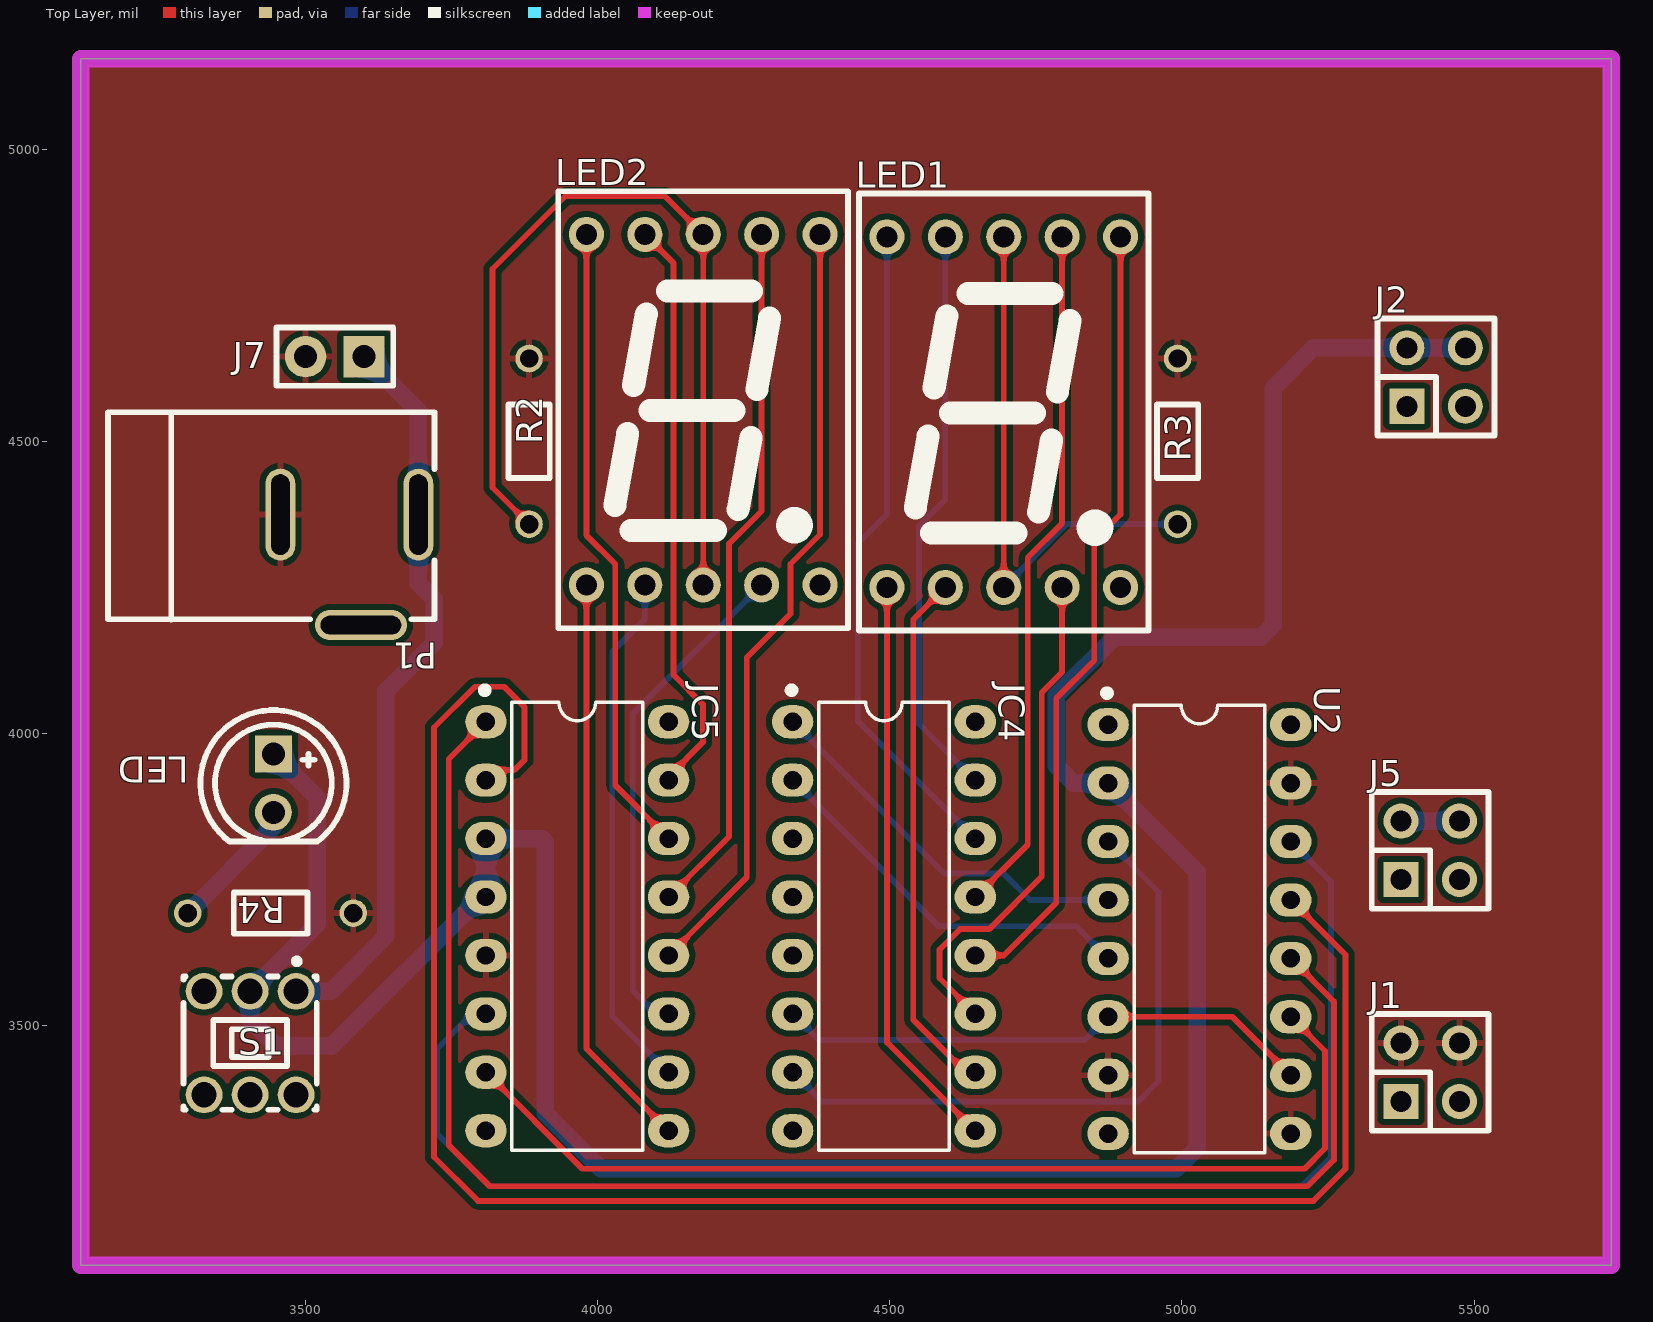
[diagram p0: Top Layer view]
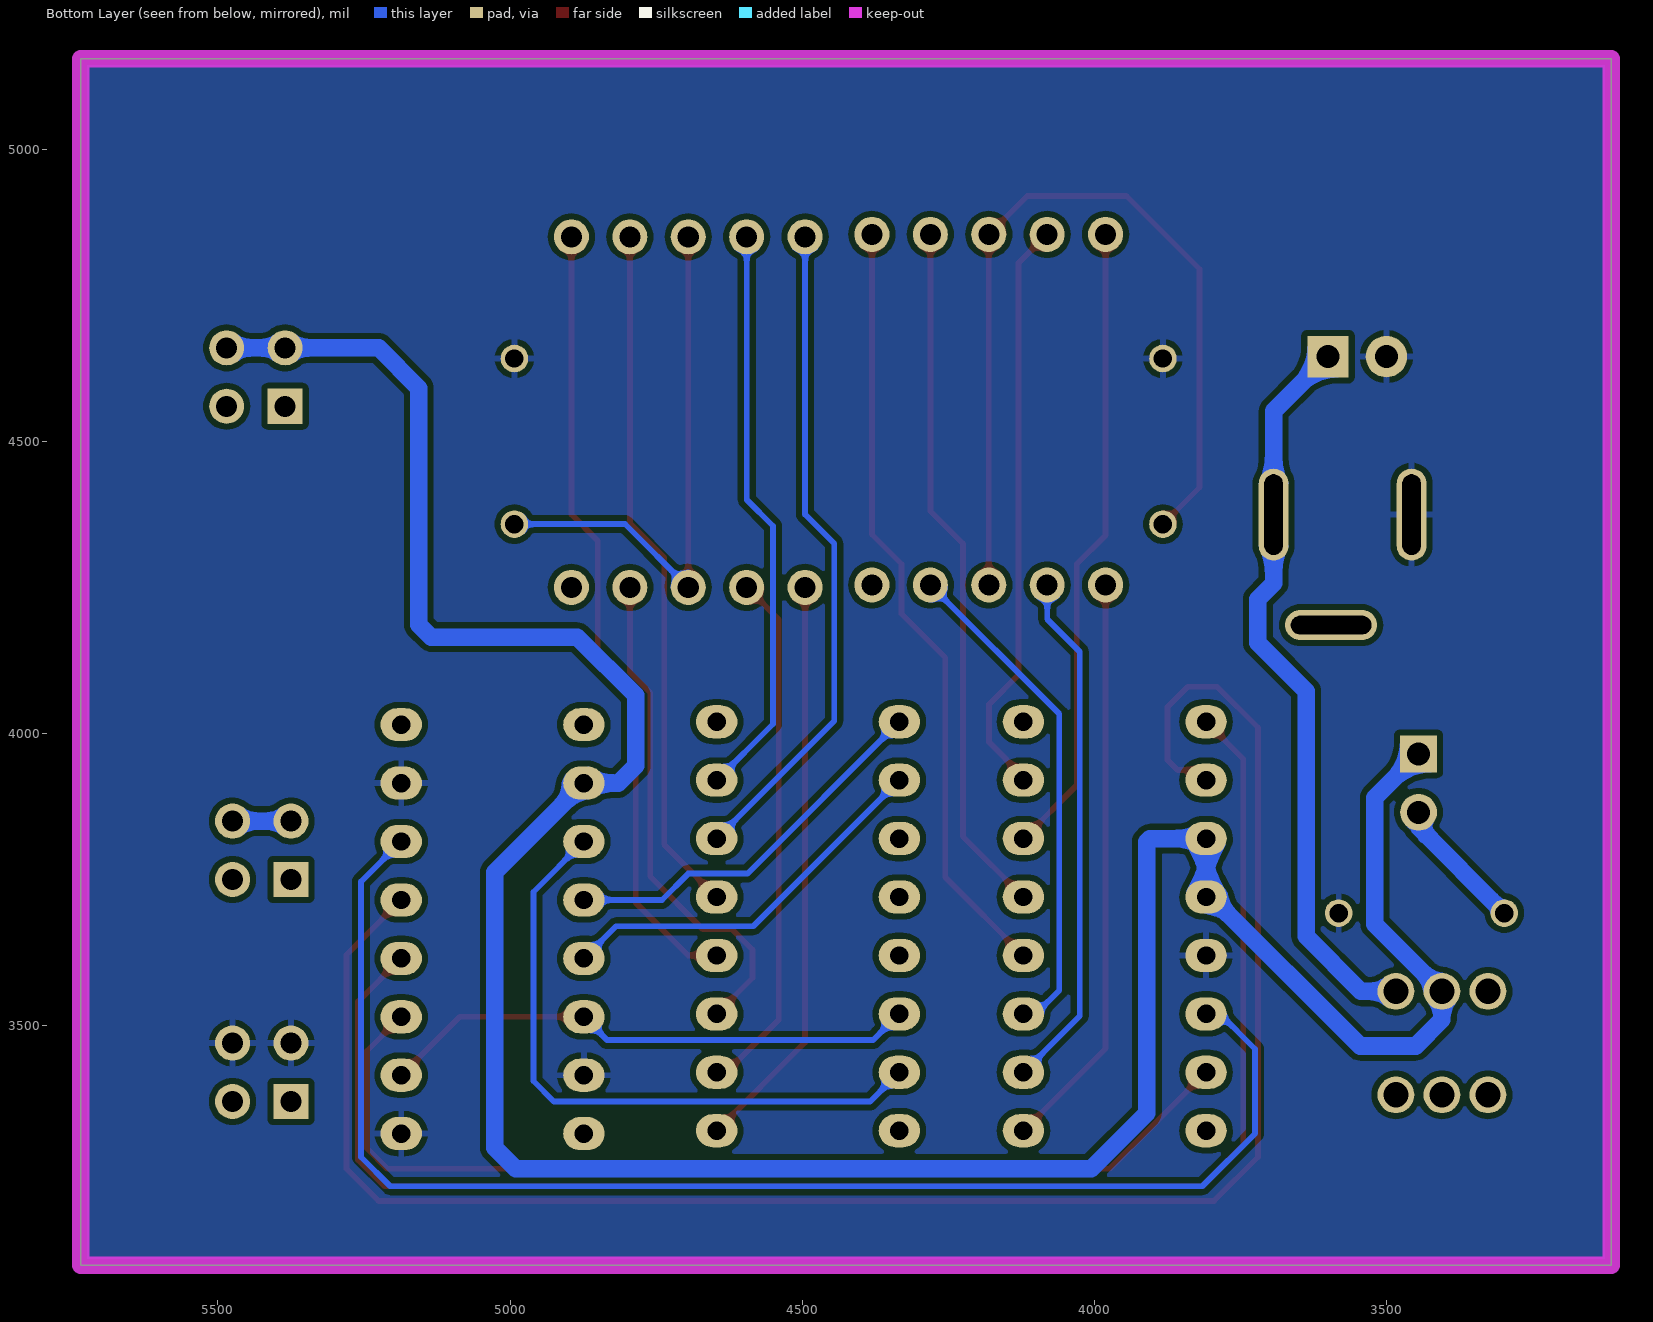
[diagram p1: Bottom Layer view, seen from below]
# Altium PCB MISC51364.pcbdoc
Units mil, origin at the board's own origin, x right, y up, seen from the top; angles counter-clockwise.
Board outline 2620 x 2065 mil, 2 copper layers (Top Layer, Bottom Layer), stack 62.206 mil thick; 15 components, 30 nets, 99 pads, 0 vias.

## Layer stack, top to bottom
Top Solder Mask Layer: solder mask 0.394, Dk 3.3
Top Layer: signal copper 1.379
Dielectric1: surface 59.449, FR4, Dk 4.5
Bottom Layer: signal copper 1.378
Bottom Solder Mask Layer: solder mask 0.394, Dk 3.3

## Board outline
3115,5155 3115,3090 5735,3090 5735,5155

## Design rules (kind name [scope] priority, off if disabled: settings)
BoardOutlineClearance copperThickness2oz_1 [All] p2 off: genericclearance=7.99 ignorepadtopadclearanceinfootprint=FALSE except(0: Arc-SplitContinuation Track-SplitContinuation SMDPad-SplitContinuation THPad-SplitContinuation Via-SplitContinuation Fill-SplitContinuation Region-SplitContinuation Poly-SplitContinuation Text-SplitContinuation Hole-SplitContinuation; 5.98: Arc-CutoutEdge Track-CutoutEdge SMDPad-CutoutEdge THPad-CutoutEdge Via-CutoutEdge Text-CutoutEdge; 6.9: Hole-OutlineEdge Hole-CutoutEdge; 10: Poly-OutlineEdge Poly-CutoutEdge; 11.81: Arc-OutlineEdge Track-OutlineEdge SMDPad-OutlineEdge THPad-OutlineEdge Via-OutlineEdge Fill-OutlineEdge Region-OutlineEdge Text-OutlineEdge Fill-CutoutEdge Region-CutoutEdge)
BoardOutlineClearance Plane_innerPlane_1 [All] p4 off: genericclearance=4.02 ignorepadtopadclearanceinfootprint=FALSE except(0: Arc-SplitContinuation Track-SplitContinuation SMDPad-SplitContinuation THPad-SplitContinuation Via-SplitContinuation Fill-SplitContinuation Region-SplitContinuation Poly-SplitContinuation Text-SplitContinuation Hole-SplitContinuation; 5.98: Arc-CutoutEdge Track-CutoutEdge SMDPad-CutoutEdge THPad-CutoutEdge Via-CutoutEdge Text-CutoutEdge; 6.9: Hole-OutlineEdge Hole-CutoutEdge; 10: Poly-OutlineEdge Poly-CutoutEdge; 11.81: Arc-OutlineEdge Track-OutlineEdge SMDPad-OutlineEdge THPad-OutlineEdge Via-OutlineEdge Fill-OutlineEdge Region-OutlineEdge Text-OutlineEdge Fill-CutoutEdge Region-CutoutEdge)
BoardOutlineClearance Copper_copperRegion_1 [All] p6 off: genericclearance=4.02 ignorepadtopadclearanceinfootprint=FALSE except(0: Arc-SplitContinuation Track-SplitContinuation SMDPad-SplitContinuation THPad-SplitContinuation Via-SplitContinuation Fill-SplitContinuation Region-SplitContinuation Poly-SplitContinuation Text-SplitContinuation Hole-SplitContinuation; 5.98: Arc-CutoutEdge Track-CutoutEdge SMDPad-CutoutEdge THPad-CutoutEdge Via-CutoutEdge Text-CutoutEdge; 6.9: Hole-OutlineEdge Hole-CutoutEdge; 10: Poly-OutlineEdge Poly-CutoutEdge; 11.81: Arc-OutlineEdge Track-OutlineEdge SMDPad-OutlineEdge THPad-OutlineEdge Via-OutlineEdge Fill-OutlineEdge Region-OutlineEdge Text-OutlineEdge Fill-CutoutEdge Region-CutoutEdge)
BoardOutlineClearance copperThickness1oz_1 [All] p8: genericclearance=4.02 ignorepadtopadclearanceinfootprint=FALSE except(0: Arc-SplitContinuation Track-SplitContinuation SMDPad-SplitContinuation THPad-SplitContinuation Via-SplitContinuation Fill-SplitContinuation Region-SplitContinuation Poly-SplitContinuation Text-SplitContinuation Hole-SplitContinuation; 5.98: Arc-CutoutEdge Track-CutoutEdge SMDPad-CutoutEdge THPad-CutoutEdge Via-CutoutEdge Text-CutoutEdge; 6.9: Hole-OutlineEdge Hole-CutoutEdge; 10: Poly-OutlineEdge Poly-CutoutEdge; 11.81: Arc-OutlineEdge Track-OutlineEdge SMDPad-OutlineEdge THPad-OutlineEdge Via-OutlineEdge Fill-OutlineEdge Region-OutlineEdge Text-OutlineEdge Fill-CutoutEdge Region-CutoutEdge)
Clearance copperThickness2oz [All] p1 off: gap=7.99 ignorepadtopadclearanceinfootprint=FALSE except(5.98: SMDPad-Track SMDPad-SMDPad THPad-Track SMDPad-THPad THPad-THPad Track-Via SMDPad-Via THPad-Via Via-Via Fill-SMDPad Region-SMDPad Fill-THPad Region-THPad Fill-Via Region-Via Fill-Fill Fill-Region Region-Region Arc-Track Arc-SMDPad Arc-THPad Arc-Via Fill-Arc Region-Arc Arc-Arc Text-Track SMDPad-Text Text-THPad Text-Via Fill-Text Region-Text Arc-Text Text-Text; 6.9: Hole-Track Hole-SMDPad Hole-THPad Hole-Via Fill-Hole Region-Hole Hole-Arc Hole-Text; 10: Poly-Track Poly-SMDPad Poly-THPad Poly-Via Poly-Fill Poly-Region Poly-Poly Poly-Arc Poly-Text Poly-Hole; 11.81: Fill-Track Region-Track)
Clearance Plane_innerPlane [All] p3 off: gap=4.02 ignorepadtopadclearanceinfootprint=FALSE except(5.98: SMDPad-Track SMDPad-SMDPad THPad-Track SMDPad-THPad THPad-THPad Track-Via SMDPad-Via THPad-Via Via-Via Fill-SMDPad Region-SMDPad Fill-THPad Region-THPad Fill-Via Region-Via Fill-Fill Fill-Region Region-Region Arc-Track Arc-SMDPad Arc-THPad Arc-Via Fill-Arc Region-Arc Arc-Arc Text-Track SMDPad-Text Text-THPad Text-Via Fill-Text Region-Text Arc-Text Text-Text; 6.9: Hole-Track Hole-SMDPad Hole-THPad Hole-Via Fill-Hole Region-Hole Hole-Arc Hole-Text; 10: Poly-Track Poly-SMDPad Poly-THPad Poly-Via Poly-Fill Poly-Region Poly-Poly Poly-Arc Poly-Text Poly-Hole; 11.81: Fill-Track Region-Track)
Clearance Copper_copperRegion [All] p5 off: gap=4.02 ignorepadtopadclearanceinfootprint=FALSE except(5.98: SMDPad-Track SMDPad-SMDPad THPad-Track SMDPad-THPad THPad-THPad Track-Via SMDPad-Via THPad-Via Via-Via Fill-SMDPad Region-SMDPad Fill-THPad Region-THPad Fill-Via Region-Via Fill-Fill Fill-Region Region-Region Arc-Track Arc-SMDPad Arc-THPad Arc-Via Fill-Arc Region-Arc Arc-Arc Text-Track SMDPad-Text Text-THPad Text-Via Fill-Text Region-Text Arc-Text Text-Text; 6.9: Hole-Track Hole-SMDPad Hole-THPad Hole-Via Fill-Hole Region-Hole Hole-Arc Hole-Text; 10: Poly-Track Poly-SMDPad Poly-THPad Poly-Via Poly-Fill Poly-Region Poly-Poly Poly-Arc Poly-Text Poly-Hole; 11.81: Fill-Track Region-Track)
Clearance copperThickness1oz [All] p7: gap=4.02 ignorepadtopadclearanceinfootprint=FALSE except(5.98: SMDPad-Track SMDPad-SMDPad THPad-Track SMDPad-THPad THPad-THPad Track-Via SMDPad-Via THPad-Via Via-Via Fill-SMDPad Region-SMDPad Fill-THPad Region-THPad Fill-Via Region-Via Fill-Fill Fill-Region Region-Region Arc-Track Arc-SMDPad Arc-THPad Arc-Via Fill-Arc Region-Arc Arc-Arc Text-Track SMDPad-Text Text-THPad Text-Via Fill-Text Region-Text Arc-Text Text-Text; 6.9: Hole-Track Hole-SMDPad Hole-THPad Hole-Via Fill-Hole Region-Hole Hole-Arc Hole-Text; 10: Poly-Track Poly-SMDPad Poly-THPad Poly-Via Poly-Fill Poly-Region Poly-Poly Poly-Arc Poly-Text Poly-Hole; 11.81: Fill-Track Region-Track)
DiffPairsRouting differentialPair [All] p1: maxlimit=6 minlimit=6 mostfreqgap=6 toplayer_minwidth=5 toplayer_prefwidth=10 toplayer_maxwidth=100 toplayer_mingap=6 toplayer_prefgap=6 toplayer_maxgap=6 bottomlayer_minwidth=5 bottomlayer_prefwidth=10 bottomlayer_maxwidth=100 bottomlayer_mingap=6 bottomlayer_prefgap=6 bottomlayer_maxgap=6 maxuncoupledlength=10
HoleToHoleClearance otherClearance [All] p1: gap=11.81 allowstackedmicrovias=TRUE
Length netLength [All] p1: minlimit=0 maxlimit=0
PasteMaskExpansion pasteMaskExpansion [All] p1: expansion=0
PlaneConnect innerPlane [All] p1: planeconnectstyle=Relief reliefexpansion=20 reliefentries=4 reliefconductorwidth=10 reliefairgap=10
PolygonConnect copperRegion [All] p1: connectstyle=Relief reliefconductorwidth=10 reliefentries=4 polygonreliefangle="90 Angle" airgapwidth=10 via.connectstyle=Relief via.reliefconductorwidth=10 via.reliefentries=4 via.polygonreliefangle="90 Angle" via.airgapwidth=10
RoutingVias viaSize [All] p1: holewidth=12.01 width=24.02 viastyle="Through Hole" minholewidth=11.81 minwidth=19.68 maxholewidth=248.03 maxwidth=393.7
SolderMaskExpansion solderMaskExpansion [IsVia] p1: expansion=-1000 istentingtop=TRUE
SolderMaskExpansion solderMaskExpansion [All] p2: expansion=2 istentingtop=FALSE
Width copperThickness2oz_2 [All] p1 off: maxlimit=100 minlimit=8 preferedwidth=10
Width copperThickness1oz_2 [All] p2: maxlimit=100 minlimit=5 preferedwidth=10

## Components (designator, comment, footprint, x,y, rotation, side; value= is the part's Value field where it differs from the comment)
J1 "" HDR-TH_4P-P2.54-V-M-R2-C2-S2.54-1 5425,3420 r0 top
J2 "" HDR-TH_4P-P2.54-V-M-R2-C2-S2.54-1 5435,4610 r0 top
J5 "" HDR-TH_4P-P2.54-V-M-R2-C2-S2.54-1 5425,3800 r0 top
J7 "" HDR-TH_2P-P2.54-V-M-1 3550,4645 r180 top
JC4 "CD74HCT4511E" PDIP-16_L19.3-W6.4-P2.54-LS7.94-BL 4490,3670 r270 top
JC5 "CD74HCT4511E" PDIP-16_L19.3-W6.4-P2.54-LS7.94-BL 3965,3670 r270 top
LED "" LED-TH_5mm 3445,3915 r270 top
LED1 "" LED-SEG-TH_10P-L12.6-W19.0-P2.54-S15.24-BL 4695,4550 r0 top
LED2 "" LED-SEG-TH_10P-L12.6-W19.0-P2.54-S15.24-BL 4180.63,4554.13 r0 top
P1 "" DC-2.0 3570,4385 r180 top
R2 "1kΩ" Res_1/8W 3885,4500 r90 top
R3 "1kΩ" Res_1/8W 4995,4500 r90 top
R4 "1kΩ" Res_1/8W 3440,3695 r180 top
S1 "自锁开关 5.8Z白灰白260G" SW-TH_6P-L5.8-W5.8-P2.00-LS4.5-TR 3405,3470 r0 top
U2 "4518BDM" PDIP-16_L19.3-W6.4-P2.54-LS7.94-BL 5030,3665 r270 top

## Footprints (in the part's own frame and the unit in brackets; to place one, negate y for a bottom-side part, rotate by r counter-clockwise, add the part's x,y. Pads: shape width x height; smd on the part's side, far side on the other; paste and mask are expansions set on the pad)
DC-2.0 [mil]
  oval 157.5x51.2 hole 31.5 slot 137.8 at 0 deg paste+0 mask+2: 2(-24.7,199.5)
  oval 51.2x157.5 hole 31.5 slot 137.8 at 90 deg paste+0 mask+2: 3(113.1,10.5) 4(-123.1,10.5)
  silkscreen extent -151,-165 408,190
HDR-TH_2P-P2.54-V-M-1 [mm]
  rect 1.8x1.8 hole 1: 1(-1.27,0)
  round 1.8 hole 1: 2(1.27,0)
  silkscreen extent -2.54,-1.27 2.54,1.27
HDR-TH_4P-P2.54-V-M-R2-C2-S2.54-1 [mil]
  rect 60x60 hole 36: 1(-50,-50)
  round 60 hole 36: 2(-50,50) 3(50,-50) 4(50,50)
  silkscreen extent -100,-100 100,100
LED-SEG-TH_10P-L12.6-W19.0-P2.54-S15.24-BL [mil]
  round 60 hole 36: 1(-200,-300) 2(-100,-300) 3(0,-300) 4(100,-300) 5(200,-300) 6(200,300) 7(100,300) 8(0,300) 9(-100,300) 10(-200,300)
  silkscreen extent -248,-374 248,374
LED-TH_5mm [mm]
  rect 1.6x1.6 hole 1 paste+0 mask+0.051: 1(-1.27,0)
  round 1.6 hole 1 paste+0 mask+0.051: 2(1.27,0)
  silkscreen extent -3.17,-3.17 2.54,3.17
PDIP-16_L19.3-W6.4-P2.54-LS7.94-BL [mm]
  oval 1.44x1.8 hole 0.8: 1(-8.89,-3.97) 2(-6.35,-3.97) 3(-3.81,-3.97) 4(-1.27,-3.97) 5(1.27,-3.97) 6(3.81,-3.97) 7(6.35,-3.97) 8(8.89,-3.97) 9(8.89,3.97) 10(6.35,3.97) 11(3.81,3.97) 12(1.27,3.97) 13(-1.27,3.97) 14(-3.81,3.97) 15(-6.35,3.97) 16(-8.89,3.97)
  silkscreen extent -10.41,-4.17 9.73,2.84
Res_1/8W [mil]
  round 47.2 hole 31.5 paste+0 mask+2: 1(-141.7,2.48) 2(141.7,2.48)
  silkscreen extent -63,-33 63,38
SW-TH_6P-L5.8-W5.8-P2.00-LS4.5-TR [mm]
  round 1.6 hole 1.1: 1(2,2.25) 2(0,2.25) 3(-2,2.25) 4(-2,-2.25) 5(0,-2.25) 6(2,-2.25)
  silkscreen extent -2.9,-2.9 2.9,3.68

## Nets (pads, with @x,y where several pads share a name; then routed paths per layer and width w, separated by ;. In a path a pad name is that pad's centre, name@x,y a point inside that pad or via, vN(x,y) a via of type N, cw(c..) or ccw(c..) an arc to the next point about the centre after c; other vN are vias at no path point)
$1N227: LED2.3 LED2.8 R2.1 | length 1502.3
  Top Layer w10: R2.1 3820,4420.82 3820,4795 3945,4920 4114.76,4920 LED2.8 LED2.3
$1N329: LED1.3 LED1.8 R3.1 | length 942.4
  Top Layer w10: LED1.3 LED1.8
  Bottom Layer w10: LED1.3 4803.3,4358.3 R3.1
$1N1315: J7.1 P1.4 S1.1 | length 1269
  Bottom Layer w30: S1.1 3543.58,3558.58 3637.5,3652.5 3637.5,4072.5 3720,4155 3720,4230 3693.1,4256.9 P1.4 3693.1,4551.9 J7.1
$1N1556: LED.2 R4.2 | length 233.2
  Bottom Layer w30: R4.2 3445,3839.22 LED.2
$1N1841: JC5.13 LED2.7 | length 1200.1
  Top Layer w10: JC5.13 4225,3823.7 4225,4325 4280.63,4380.63 LED2.7
$1N1846: JC5.12 LED2.6 | length 1341.6
  Top Layer w10: JC5.12 4255,3753.7 4255,4130 4330,4205 4330,4290 4380.63,4340.63 LED2.6
$1N1852: JC5.11 LED2.4 | length 863.4
  Bottom Layer w10: JC5.11 4100,3520 4060,3560 4060,4033.51 LED2.4
$1N1858: JC5.10 LED2.2 | length 897.1
  Bottom Layer w10: LED2.2 4080.63,4195.63 4025,4140 4025,3516.3 JC5.10
$1N1864: JC5.9 LED2.1 | length 992.4
  Top Layer w10: LED2.1 3980.63,3460.67 JC5.9
$1N1870: JC5.15 LED2.9 | length 999.6
  Top Layer w10: LED2.9 4130,4804.76 4130,4100 4180,4050 4180,3985 4121.3,3926.3 JC5.15
$1N1876: JC5.14 LED2.10 | length 1092.4
  Top Layer w10: LED2.10 3980.63,4339.37 4030,4290 4030,3911.3 JC5.14
$1N1882: JC4.13 LED1.7 | length 1191.6
  Top Layer w10: JC4.13 4735.98,3809.68 4735.98,4300.98 4795,4360 LED1.7
$1N1887: JC4.12 LED1.6 | length 1361.5
  Top Layer w10: JC4.12 4695,3620 4785,3710 4785,4060 4850,4125 4850,4330 4895,4375 LED1.6
$1N1892: JC4.11 LED1.4 | length 871.7
  Top Layer w10: JC4.11 4585,3581.3 4585,3630 4620,3665 4670,3665 4760,3755 4760,4070 4795,4105 LED1.4
$1N1897: JC4.10 LED1.2 | length 906.4
  Top Layer w10: LED1.2 4540,4195 4540,3510 4630,3420 JC4.10
$1N1906: JC4.9 LED1.1 | length 992.7
  Top Layer w10: LED1.1 4495,3471.3 JC4.9
$1N1912: JC4.15 LED1.9 | length 988.5
  Bottom Layer w10: LED1.9 4595,4400 4550,4355 4550,4016.3 JC4.15
$1N1918: JC4.14 LED1.10 | length 1134.1
  Bottom Layer w10: LED1.10 4495,4375 4445,4325 4445,4021.3 JC4.14
$1N1947: JC5.7 U2.11 | length 1768.5
  Top Layer w10: JC5.7 3973.7,3255 5210,3255 5245,3290 5245,3456.3 U2.11
$1N1953: JC5.6 U2.14 | length 2410
  Bottom Layer w10: JC5.6 3785,3520 3725,3460 3725,3315 3815,3225 5205,3225 5255,3275 5255,3746.3 U2.14
$1N1959: JC5.2 U2.13 | length 3216.9
  Top Layer w10: JC5.2 3826.63,3937.93 3857.93,3937.93 3875,3955 3875,4045 3840,4080 3790,4080 3720,4010 3720,3275 3795,3200 5225,3200 5280,3255 5280,3621.3 U2.13
$1N1965: JC5.1 U2.12 | length 2689.5
  Top Layer w10: JC5.1 3745,3956.3 3745,3295 3815,3225 5215,3225 5260,3270 5260,3541.3 U2.12
$1N2098: JC4.6 U2.6 U2.10 | length 929.2
  Top Layer w10: U2.6 5086.3,3515 U2.10
  Bottom Layer w10: JC4.6 4378.7,3475 4833.7,3475 U2.6
$1N2106: JC4.7 U2.3 | length 1107.3
  Bottom Layer w10: JC4.7 4383.7,3370 4925,3370 4960,3405 4960,3728.7 U2.3
$1N2111: JC4.1 U2.4 | length 666.3
  Bottom Layer w10: JC4.1 4593.7,3760 4695,3760 4740,3715 U2.4
$1N2117: JC4.2 U2.5 | length 666.3
  Bottom Layer w10: JC4.2 4583.7,3670 4818.7,3670 U2.5
CP: J5.2 J5.4 | length 100
  Bottom Layer w30: J5.2 J5.4
GND: J1.2 J1.4 J7.2 JC5.5 P1.3 R2.2 R3.2 R4.1 U2.7 U2.9 U2.15
JC3: U2.1
VCC: J2.2 J2.4 JC5.3 JC5.4 LED.1 S1.2 U2.2 | length 4992.4
  Bottom Layer w30: LED.1 3520,3890 3520,3673.58 S1.2 3405,3510 3450,3465 3545,3465 3800,3720 JC5.4 JC5.3 3905,3820 3910,3815 3910,3350 4005,3255 4990,3255 5026.21,3291.21 5026.21,3762.49 U2.2 4815,3915 4785,3945 4785,4065 4885,4165 5135,4165 5156.21,4186.21 5156.21,4591.21 5225,4660 J2.2 J2.4
pads on no net: J1.1 J1.3 J2.1 J2.3 J5.1 J5.3 JC4.3 JC4.4 JC4.5 JC4.8 JC4.16 JC5.8 JC5.16 LED1.5 LED2.5 P1.2 S1.3 S1.4 S1.5 S1.6 U2.8 U2.16

## Polygon pours and split planes (outlines as drawn)
GND on Top Layer (solid, remove dead copper, pour order 0): 3030,5255 3030,3010 5825,3010 5825,5255
GND on Bottom Layer (solid, remove dead copper, pour order 2): 3000,5325 3000,3000 5800,3000 5800,5325

## Keep-outs
Board Outline Layer:
  the board outline again, w30

## Other copper
Top Layer:
  region net $1N1876: 3985.63,4813.13 3975.63,4813.13 3975.53,4815.41 3975.24,4817.38 3974.77,4819.08 3974.13,4820.54 3973.35,4821.82 3972.42,4822.94 3970.2,4824.88 3964.64,4828.59 3961.5,4830.98 3959.89,4832.44 3958.26,4834.13 4002.99,4834.13 4001.36,4832.44 3999.75,4830.98 3996.61,4828.59 3991.05,4824.88 3988.83,4822.94 3987.9,4821.82 3987.12,4820.54 3986.48,4819.08 3986.02,4817.38 3985.73,4815.41
  region net $1N1876: 4084.35,3849.88 4094.54,3853.83 4096.02,3852.53 4097.75,3851.32 4099.67,3850.24 4101.72,3849.32 4103.83,3848.6 4105.95,3848.12 4108.01,3847.91 4109.95,3848.02 4089.42,3833.75 4090.28,3835.86 4090.57,3837.99 4090.37,3840.12 4089.74,3842.22 4088.75,3844.27 4087.48,3846.24 4085.99,3848.12
  region net $1N1870: 4113.15,4828.68 4106.08,4821.61 4104.4,4823.15 4102.81,4824.33 4101.27,4825.2 4099.79,4825.79 4098.33,4826.14 4096.88,4826.28 4093.94,4826.07 4087.38,4824.77 4083.48,4824.24 4081.3,4824.13 4078.96,4824.18 4110.58,4855.8 4110.63,4853.46 4110.52,4851.28 4109.99,4847.38 4108.68,4840.82 4108.48,4837.88 4108.62,4836.43 4108.97,4834.97 4109.56,4833.49 4110.43,4831.95 4111.61,4830.36
  region net $1N1870: 4142.94,3955.01 4155.74,3953.67 4153.91,3951.78 4152.23,3949.83 4150.78,3947.85 4149.67,3945.83 4149.01,3943.79 4148.87,3942.76 4148.88,3941.73 4149.04,3940.69 4149.38,3939.66 4149.9,3938.62 4150.62,3937.58 4128.39,3948.35 4130.23,3948.5 4132.18,3948.92 4134.18,3949.58 4136.18,3950.43 4138.11,3951.44 4139.92,3952.56 4141.55,3953.77
  region net $1N227: 4148.1,4879.59 4155.17,4886.66 4156.85,4885.12 4158.45,4883.94 4159.98,4883.07 4161.46,4882.48 4162.92,4882.13 4164.37,4881.99 4167.31,4882.19 4173.87,4883.5 4177.77,4884.03 4179.95,4884.13 4182.29,4884.09 4150.67,4852.46 4150.62,4854.81 4150.73,4856.99 4151.26,4860.89 4152.57,4867.45 4152.77,4870.39 4152.63,4871.84 4152.28,4873.3 4151.69,4874.78 4150.82,4876.31 4149.64,4877.91
  region net $1N227: 3856.18,4377.57 3863.25,4384.64 3864.48,4383.52 3865.67,4382.63 3866.82,4381.95 3867.96,4381.46 3870.21,4380.97 3872.51,4380.95 3877.58,4381.58 3880.52,4381.86 3883.84,4381.86 3858.96,4356.99 3858.96,4360.3 3859.24,4363.24 3859.88,4368.31 3859.86,4370.61 3859.36,4372.86 3858.87,4374 3858.2,4375.16 3857.31,4376.34
  region net $1N227: 4175.63,4295.13 4185.63,4295.13 4185.73,4292.86 4186.02,4290.89 4186.48,4289.19 4187.12,4287.72 4187.9,4286.45 4188.83,4285.33 4191.05,4283.39 4196.61,4279.68 4199.75,4277.29 4201.36,4275.83 4202.99,4274.13 4158.26,4274.13 4159.89,4275.83 4161.5,4277.29 4164.64,4279.68 4170.2,4283.39 4172.42,4285.33 4173.35,4286.45 4174.13,4287.72 4174.77,4289.19 4175.24,4290.89 4175.53,4292.86
  region net $1N227: 4185.63,4813.13 4175.63,4813.13 4175.53,4815.41 4175.24,4817.38 4174.77,4819.08 4174.13,4820.54 4173.35,4821.82 4172.42,4822.94 4170.2,4824.88 4164.64,4828.59 4161.5,4830.98 4159.89,4832.44 4158.26,4834.13 4202.99,4834.13 4201.36,4832.44 4199.75,4830.98 4196.61,4828.59 4191.05,4824.88 4188.83,4822.94 4187.9,4821.82 4187.12,4820.54 4186.48,4819.08 4186.02,4817.38 4185.73,4815.41
  region net $1N1841: 4285.63,4813.13 4275.63,4813.13 4275.53,4815.41 4275.24,4817.38 4274.77,4819.08 4274.13,4820.54 4273.35,4821.82 4272.42,4822.94 4270.2,4824.88 4264.64,4828.59 4261.5,4830.98 4259.89,4832.44 4258.26,4834.13 4302.99,4834.13 4301.36,4832.44 4299.75,4830.98 4296.61,4828.59 4291.05,4824.88 4288.83,4822.94 4287.9,4821.82 4287.12,4820.54 4286.48,4819.08 4286.02,4817.38 4285.73,4815.41
  region net $1N1841: 4148.06,3753.83 4158.25,3749.88 4156.61,3748.12 4155.12,3746.24 4153.85,3744.27 4152.86,3742.22 4152.23,3740.12 4152.03,3737.99 4152.32,3735.86 4153.18,3733.75 4132.65,3748.02 4134.59,3747.91 4136.65,3748.12 4138.77,3748.6 4140.88,3749.32 4142.93,3750.24 4144.85,3751.32 4146.58,3752.53
  region net $1N1846: 4385.63,4813.13 4375.63,4813.13 4375.53,4815.41 4375.24,4817.38 4374.77,4819.08 4374.13,4820.54 4373.35,4821.82 4372.42,4822.94 4370.2,4824.88 4364.64,4828.59 4361.5,4830.98 4359.89,4832.44 4358.26,4834.13 4402.99,4834.13 4401.36,4832.44 4399.75,4830.98 4396.61,4828.59 4391.05,4824.88 4388.83,4822.94 4387.9,4821.82 4387.12,4820.54 4386.48,4819.08 4386.02,4817.38 4385.73,4815.41
  region net $1N1846: 4148.06,3653.83 4158.25,3649.88 4156.61,3648.12 4155.12,3646.24 4153.85,3644.27 4152.86,3642.22 4152.23,3640.12 4152.03,3637.99 4152.32,3635.86 4153.18,3633.75 4132.65,3648.02 4134.59,3647.91 4136.65,3648.12 4138.77,3648.6 4140.88,3649.32 4142.93,3650.24 4144.85,3651.32 4146.58,3652.53
  region net $1N1864: 3985.63,4213.13 3975.63,4213.13 3975.53,4215.41 3975.24,4217.38 3974.77,4219.08 3974.13,4220.54 3973.35,4221.82 3972.42,4222.94 3970.2,4224.88 3964.64,4228.59 3961.5,4230.98 3959.89,4232.44 3958.26,4234.13 4002.99,4234.13 4001.36,4232.44 3999.75,4230.98 3996.61,4228.59 3991.05,4224.88 3988.83,4222.94 3987.9,4221.82 3987.12,4220.54 3986.48,4219.08 3986.02,4217.38 3985.73,4215.41
  region net $1N1864: 4084.35,3349.88 4094.54,3353.83 4096.02,3352.53 4097.75,3351.32 4099.67,3350.24 4101.72,3349.32 4103.83,3348.6 4105.95,3348.12 4108.01,3347.91 4109.95,3348.02 4089.42,3333.75 4090.28,3335.86 4090.57,3337.99 4090.37,3340.12 4089.74,3342.22 4088.75,3344.27 4087.48,3346.24 4085.99,3348.12
  region net $1N329: 4700,4809 4690,4809 4689.9,4811.27 4689.61,4813.24 4689.14,4814.94 4688.51,4816.41 4687.72,4817.69 4686.8,4818.81 4684.57,4820.74 4679.01,4824.46 4675.88,4826.85 4674.26,4828.31 4672.64,4830 4717.36,4830 4715.74,4828.31 4714.12,4826.85 4710.99,4824.46 4705.43,4820.74 4703.2,4818.81 4702.28,4817.69 4701.49,4816.41 4700.86,4814.94 4700.39,4813.24 4700.1,4811.27
  region net $1N329: 4690,4291 4700,4291 4700.1,4288.73 4700.39,4286.76 4700.86,4285.06 4701.49,4283.59 4702.28,4282.31 4703.2,4281.19 4705.43,4279.26 4710.99,4275.54 4714.12,4273.15 4715.74,4271.69 4717.36,4270 4672.64,4270 4674.26,4271.69 4675.88,4273.15 4679.01,4275.54 4684.57,4279.26 4686.8,4281.19 4687.72,4282.31 4688.51,4283.59 4689.14,4285.06 4689.61,4286.76 4689.9,4288.73
  region net $1N1882: 4800,4809 4790,4809 4789.9,4811.27 4789.61,4813.24 4789.14,4814.94 4788.51,4816.41 4787.72,4817.69 4786.8,4818.81 4784.57,4820.74 4779.01,4824.46 4775.88,4826.85 4774.26,4828.31 4772.64,4830 4817.36,4830 4815.74,4828.31 4814.12,4826.85 4810.99,4824.46 4805.43,4820.74 4803.2,4818.81 4802.28,4817.69 4801.49,4816.41 4800.86,4814.94 4800.39,4813.24 4800.1,4811.27
  region net $1N1887: 4900,4809 4890,4809 4889.9,4811.27 4889.61,4813.24 4889.14,4814.94 4888.51,4816.41 4887.72,4817.69 4886.8,4818.81 4884.57,4820.74 4879.01,4824.46 4875.88,4826.85 4874.26,4828.31 4872.64,4830 4917.36,4830 4915.74,4828.31 4914.12,4826.85 4910.99,4824.46 4905.43,4820.74 4903.2,4818.81 4902.28,4817.69 4901.49,4816.41 4900.86,4814.94 4900.39,4813.24 4900.1,4811.27
  region net $1N1887: 4693.83,3625 4693.83,3615 4691.66,3614.89 4689.45,3614.54 4687.25,3613.97 4685.14,3613.15 4683.18,3612.1 4681.43,3610.81 4679.96,3609.28 4678.83,3607.5 4678.83,3632.5 4679.96,3630.72 4681.43,3629.19 4683.18,3627.9 4685.14,3626.85 4687.25,3626.03 4689.45,3625.46 4691.66,3625.11
  region net $1N1892: 4609.35,3549.88 4619.54,3553.83 4621.02,3552.53 4622.75,3551.32 4624.67,3550.24 4626.72,3549.32 4628.83,3548.6 4630.95,3548.12 4633.01,3547.91 4634.95,3548.02 4614.42,3533.75 4615.28,3535.86 4615.57,3537.99 4615.37,3540.12 4614.74,3542.22 4613.75,3544.27 4612.48,3546.24 4610.99,3548.12
  region net $1N1892: 4800,4209 4790,4209 4789.9,4211.27 4789.61,4213.24 4789.14,4214.94 4788.51,4216.41 4787.72,4217.69 4786.8,4218.81 4784.57,4220.74 4779.01,4224.46 4775.88,4226.85 4774.26,4228.31 4772.64,4230 4817.36,4230 4815.74,4228.31 4814.12,4226.85 4810.99,4224.46 4805.43,4220.74 4803.2,4218.81 4802.28,4217.69 4801.49,4216.41 4800.86,4214.94 4800.39,4213.24 4800.1,4211.27
  region net $1N1882: 4673.06,3753.83 4683.25,3749.88 4681.61,3748.12 4680.12,3746.24 4678.85,3744.27 4677.86,3742.22 4677.23,3740.12 4677.03,3737.99 4677.32,3735.86 4678.18,3733.75 4657.65,3748.02 4659.59,3747.91 4661.65,3748.12 4663.77,3748.6 4665.88,3749.32 4667.93,3750.24 4669.85,3751.32 4671.58,3752.53
  region net $1N2098: 5149.35,3444.88 5159.54,3448.83 5161.02,3447.53 5162.75,3446.32 5164.67,3445.24 5166.72,3444.32 5168.83,3443.6 5170.95,3443.12 5173.01,3442.91 5174.95,3443.02 5154.42,3428.75 5155.28,3430.86 5155.57,3432.99 5155.37,3435.12 5154.74,3437.22 5153.75,3439.27 5152.48,3441.24 5150.99,3443.12
  region net $1N2098: 4921.23,3520 4921.23,3510 4919.06,3509.89 4916.85,3509.54 4914.65,3508.97 4912.54,3508.15 4910.58,3507.1 4908.83,3505.81 4907.36,3504.28 4906.23,3502.5 4906.23,3527.5 4907.36,3525.72 4908.83,3524.19 4910.58,3522.9 4912.54,3521.85 4914.65,3521.03 4916.85,3520.46 4919.06,3520.11
  region net $1N1947: 5223.25,3485.12 5213.06,3481.17 5211.58,3482.47 5209.85,3483.68 5207.93,3484.76 5205.88,3485.68 5203.77,3486.4 5201.65,3486.88 5199.59,3487.09 5197.65,3486.98 5218.18,3501.25 5217.32,3499.14 5217.03,3497.01 5217.23,3494.88 5217.86,3492.78 5218.85,3490.73 5220.12,3488.76 5221.61,3486.88
  region net $1N1947: 3845.65,3390.12 3835.46,3386.17 3833.98,3387.47 3832.25,3388.68 3830.33,3389.76 3828.28,3390.68 3826.17,3391.4 3824.05,3391.88 3821.99,3392.09 3820.05,3391.98 3840.58,3406.25 3839.72,3404.14 3839.43,3402.01 3839.63,3399.88 3840.26,3397.78 3841.25,3395.73 3842.52,3393.76 3844.01,3391.88
  region net $1N1965: 5223.25,3585.12 5213.06,3581.17 5211.58,3582.47 5209.85,3583.68 5207.93,3584.76 5205.88,3585.68 5203.77,3586.4 5201.65,3586.88 5199.59,3587.09 5197.65,3586.98 5218.18,3601.25 5217.32,3599.14 5217.03,3597.01 5217.23,3594.88 5217.86,3592.78 5218.85,3590.73 5220.12,3588.76 5221.61,3586.88
  region net $1N1965: 3781.94,3986.17 3771.75,3990.12 3773.39,3991.88 3774.88,3993.76 3776.15,3995.73 3777.14,3997.78 3777.77,3999.88 3777.97,4002.01 3777.68,4004.14 3776.82,4006.25 3797.35,3991.98 3795.41,3992.09 3793.35,3991.88 3791.23,3991.4 3789.12,3990.68 3787.07,3989.76 3785.15,3988.68 3783.42,3987.47
  region net $1N1959: 5223.25,3685.12 5213.06,3681.17 5211.58,3682.47 5209.85,3683.68 5207.93,3684.76 5205.88,3685.68 5203.77,3686.4 5201.65,3686.88 5199.59,3687.09 5197.65,3686.98 5218.18,3701.25 5217.32,3699.14 5217.03,3697.01 5217.23,3694.88 5217.86,3692.78 5218.85,3690.73 5220.12,3688.76 5221.61,3686.88
  region net $1N1959: 3842.59,3942.93 3857.93,3932.93 3852.05,3933 3849.36,3932.91 3847,3932.58 3845.99,3932.28 3845.11,3931.88 3844.37,3931.36 3843.79,3930.7 3843.39,3929.89 3843.18,3928.92 3843.18,3927.76 3843.4,3926.41 3827.59,3945.77 3831,3944.56 3834.94,3943.67 3838.95,3943.12
  region net $1N1906: 4609.35,3349.88 4619.54,3353.83 4621.02,3352.53 4622.75,3351.32 4624.67,3350.24 4626.72,3349.32 4628.83,3348.6 4630.95,3348.12 4633.01,3347.91 4634.95,3348.02 4614.42,3333.75 4615.28,3335.86 4615.57,3337.99 4615.37,3340.12 4614.74,3342.22 4613.75,3344.27 4612.48,3346.24 4610.99,3348.12
  region net $1N1906: 4500,4209 4490,4209 4489.9,4211.27 4489.61,4213.24 4489.14,4214.94 4488.51,4216.41 4487.72,4217.69 4486.8,4218.81 4484.57,4220.74 4479.01,4224.46 4475.88,4226.85 4474.26,4228.31 4472.64,4230 4517.36,4230 4515.74,4228.31 4514.12,4226.85 4510.99,4224.46 4505.43,4220.74 4503.2,4218.81 4502.28,4217.69 4501.49,4216.41 4500.86,4214.94 4500.39,4213.24 4500.1,4211.27
  region net $1N1897: 4604.99,3437.94 4608,3449.08 4609.8,3447.37 4611.7,3445.82 4613.68,3444.49 4615.72,3443.47 4617.81,3442.84 4619.92,3442.66 4622.03,3443.03 4623.09,3443.43 4624.14,3444.01 4611,3422.74 4611.02,3424.63 4610.74,3426.66 4610.2,3428.76 4609.45,3430.86 4608.51,3432.9 4607.43,3434.8 4606.24,3436.51
  region net $1N1897: 4569.54,4217.47 4562.47,4224.54 4564.01,4226.22 4565.2,4227.82 4566.07,4229.35 4566.66,4230.84 4567,4232.3 4567.14,4233.74 4566.94,4236.68 4565.63,4243.24 4565.11,4247.15 4565,4249.32 4565.05,4251.67 4596.67,4220.05 4594.32,4220 4592.15,4220.11 4588.24,4220.63 4581.68,4221.94 4578.74,4222.14 4577.3,4222 4575.84,4221.66 4574.35,4221.07 4572.82,4220.2 4571.22,4219.01
Bottom Layer:
  region net $1N1858: 4085.63,4213.13 4075.63,4213.13 4075.53,4215.41 4075.24,4217.38 4074.77,4219.08 4074.13,4220.54 4073.35,4221.82 4072.42,4222.94 4070.2,4224.88 4064.64,4228.59 4061.5,4230.98 4059.89,4232.44 4058.26,4234.13 4102.99,4234.13 4101.36,4232.44 4099.75,4230.98 4096.61,4228.59 4091.05,4224.88 4088.83,4222.94 4087.9,4221.82 4087.12,4220.54 4086.48,4219.08 4086.02,4217.38 4085.73,4215.41
  region net $1N1858: 4084.35,3449.88 4094.54,3453.83 4096.02,3452.53 4097.75,3451.32 4099.67,3450.24 4101.72,3449.32 4103.83,3448.6 4105.95,3448.12 4108.01,3447.91 4109.95,3448.02 4089.42,3433.75 4090.28,3435.86 4090.57,3437.99 4090.37,3440.12 4089.74,3442.22 4088.75,3444.27 4087.48,3446.24 4085.99,3448.12
  region net $1N1852: 4255.17,4221.61 4248.1,4228.68 4249.64,4230.36 4250.82,4231.95 4251.69,4233.49 4252.28,4234.97 4252.63,4236.43 4252.77,4237.88 4252.57,4240.82 4251.26,4247.38 4250.73,4251.28 4250.62,4253.46 4250.67,4255.8 4282.29,4224.18 4279.95,4224.13 4277.77,4224.24 4273.87,4224.77 4267.31,4226.07 4264.37,4226.28 4262.92,4226.14 4261.46,4225.79 4259.98,4225.2 4258.45,4224.33 4256.85,4223.15
  region net $1N1852: 4079.28,3533.65 4080.08,3546.99 4081.99,3545.13 4083.95,3543.42 4085.93,3541.94 4087.94,3540.82 4089.98,3540.14 4091,3540 4092.02,3540.02 4093.05,3540.2 4094.08,3540.55 4095.11,3541.09 4096.14,3541.84 4085.88,3519.04 4085.69,3520.83 4085.23,3522.77 4084.56,3524.8 4083.71,3526.84 4082.72,3528.82 4081.62,3530.66 4080.46,3532.3
  region net $1N329: 4720.46,4282.53 4727.53,4275.46 4725.99,4273.78 4724.8,4272.18 4723.93,4270.65 4723.34,4269.16 4723,4267.7 4722.86,4266.26 4723.06,4263.32 4724.37,4256.76 4724.89,4252.85 4725,4250.68 4724.95,4248.33 4693.33,4279.95 4695.68,4280 4697.85,4279.89 4701.76,4279.37 4708.32,4278.06 4711.26,4277.86 4712.7,4278 4714.16,4278.34 4715.65,4278.93 4717.18,4279.8 4718.78,4280.99
  region net $1N329: 4960.27,4353.3 4960.27,4363.3 4961.93,4363.37 4963.4,4363.58 4964.7,4363.92 4965.85,4364.38 4967.79,4365.62 4969.43,4367.23 4972.57,4371.27 4974.45,4373.54 4976.79,4375.89 4976.79,4340.71 4974.45,4343.06 4972.57,4345.33 4969.43,4349.37 4967.79,4350.98 4965.85,4352.22 4964.7,4352.68 4963.4,4353.02 4961.93,4353.23
  region net $1N1953: 5223.25,3785.12 5213.06,3781.17 5211.58,3782.47 5209.85,3783.68 5207.93,3784.76 5205.88,3785.68 5203.77,3786.4 5201.65,3786.88 5199.59,3787.09 5197.65,3786.98 5218.18,3801.25 5217.32,3799.14 5217.03,3797.01 5217.23,3794.88 5217.86,3792.78 5218.85,3790.73 5220.12,3788.76 5221.61,3786.88
  region net $1N1953: 3766.2,3494.13 3766.46,3508.53 3767.62,3509.84 3768.78,3511.44 3770.92,3515.19 3772.57,3519.17 3773.11,3521.06 3773.4,3522.79 3782.17,3499.38 3781.16,3500.21 3780.15,3500.82 3779.14,3501.22 3778.14,3501.43 3777.13,3501.46 3776.13,3501.32 3774.13,3500.61 3772.13,3499.42 3770.14,3497.87
  region net $1N1918: 4500,4809 4490,4809 4489.9,4811.27 4489.61,4813.24 4489.14,4814.94 4488.51,4816.41 4487.72,4817.69 4486.8,4818.81 4484.57,4820.74 4479.01,4824.46 4475.88,4826.85 4474.26,4828.31 4472.64,4830 4517.36,4830 4515.74,4828.31 4514.12,4826.85 4510.99,4824.46 4505.43,4820.74 4503.2,4818.81 4502.28,4817.69 4501.49,4816.41 4500.86,4814.94 4500.39,4813.24 4500.1,4811.27
  region net $1N1918: 4609.35,3849.88 4619.54,3853.83 4621.02,3852.53 4622.75,3851.32 4624.67,3850.24 4626.72,3849.32 4628.83,3848.6 4630.95,3848.12 4633.01,3847.91 4634.95,3848.02 4614.42,3833.75 4615.28,3835.86 4615.57,3837.99 4615.37,3840.12 4614.74,3842.22 4613.75,3844.27 4612.48,3846.24 4610.99,3848.12
  region net $1N1912: 4600,4809 4590,4809 4589.9,4811.27 4589.61,4813.24 4589.14,4814.94 4588.51,4816.41 4587.72,4817.69 4586.8,4818.81 4584.57,4820.74 4579.01,4824.46 4575.88,4826.85 4574.26,4828.31 4572.64,4830 4617.36,4830 4615.74,4828.31 4614.12,4826.85 4610.99,4824.46 4605.43,4820.74 4603.2,4818.81 4602.28,4817.69 4601.49,4816.41 4600.86,4814.94 4600.39,4813.24 4600.1,4811.27
  region net $1N1912: 4609.35,3949.88 4619.54,3953.83 4621.02,3952.53 4622.75,3951.32 4624.67,3950.24 4626.72,3949.32 4628.83,3948.6 4630.95,3948.12 4633.01,3947.91 4634.95,3948.02 4614.42,3933.75 4615.28,3935.86 4615.57,3937.99 4615.37,3940.12 4614.74,3942.22 4613.75,3944.27 4612.48,3946.24 4610.99,3948.12
  region net $1N2111: 4826.17,3710 4826.17,3720 4828.34,3720.11 4830.55,3720.46 4832.75,3721.03 4834.86,3721.85 4836.82,3722.9 4838.57,3724.19 4840.04,3725.72 4841.17,3727.5 4841.17,3702.5 4840.04,3704.28 4838.57,3705.81 4836.82,3707.1 4834.86,3708.15 4832.75,3708.97 4830.55,3709.54 4828.34,3709.89
  region net $1N2111: 4370.65,3990.12 4360.46,3986.17 4358.98,3987.47 4357.25,3988.68 4355.33,3989.76 4353.28,3990.68 4351.17,3991.4 4349.05,3991.88 4346.99,3992.09 4345.05,3991.98 4365.58,4006.25 4364.72,4004.14 4364.43,4002.01 4364.63,3999.88 4365.26,3997.78 4366.25,3995.73 4367.52,3993.76 4369.01,3991.88
  region net $1N2117: 4836.75,3644.88 4846.94,3648.83 4848.42,3647.53 4850.15,3646.32 4852.07,3645.24 4854.12,3644.32 4856.23,3643.6 4858.35,3643.12 4860.41,3642.91 4862.35,3643.02 4841.82,3628.75 4842.68,3630.86 4842.97,3632.99 4842.77,3635.12 4842.14,3637.22 4841.15,3639.27 4839.88,3641.24 4838.39,3643.12
  region net $1N2117: 4370.65,3890.12 4360.46,3886.17 4358.98,3887.47 4357.25,3888.68 4355.33,3889.76 4353.28,3890.68 4351.17,3891.4 4349.05,3891.88 4346.99,3892.09 4345.05,3891.98 4365.58,3906.25 4364.72,3904.14 4364.43,3902.01 4364.63,3899.88 4365.26,3897.78 4366.25,3895.73 4367.52,3893.76 4369.01,3891.88
  region net $1N2098: 4370.65,3490.12 4360.46,3486.17 4358.98,3487.47 4357.25,3488.68 4355.33,3489.76 4353.28,3490.68 4351.17,3491.4 4349.05,3491.88 4346.99,3492.09 4345.05,3491.98 4365.58,3506.25 4364.72,3504.14 4364.43,3502.01 4364.63,3499.88 4365.26,3497.78 4366.25,3495.73 4367.52,3493.76 4369.01,3491.88
  region net $1N2098: 4846.94,3481.17 4836.75,3485.12 4838.39,3486.88 4839.88,3488.76 4841.15,3490.73 4842.14,3492.78 4842.77,3494.88 4842.97,3497.01 4842.68,3499.14 4841.82,3501.25 4862.35,3486.98 4860.41,3487.09 4858.35,3486.88 4856.23,3486.4 4854.12,3485.68 4852.07,3484.76 4850.15,3483.68 4848.42,3482.47
  region net $1N2106: 4910.65,3785.12 4900.46,3781.17 4898.98,3782.47 4897.25,3783.68 4895.33,3784.76 4893.28,3785.68 4891.17,3786.4 4889.05,3786.88 4886.99,3787.09 4885.05,3786.98 4905.58,3801.25 4904.72,3799.14 4904.43,3797.01 4904.63,3794.88 4905.26,3792.78 4906.25,3790.73 4907.52,3788.76 4909.01,3786.88
  region net $1N2106: 4370.65,3390.12 4360.46,3386.17 4358.98,3387.47 4357.25,3388.68 4355.33,3389.76 4353.28,3390.68 4351.17,3391.4 4349.05,3391.88 4346.99,3392.09 4345.05,3391.98 4365.58,3406.25 4364.72,3404.14 4364.43,3402.01 4364.63,3399.88 4365.26,3397.78 4366.25,3395.73 4367.52,3393.76 4369.01,3391.88
  region net $1N1315: 3651.34,4614.87 3630.13,4593.66 3624.09,4597.77 3617.69,4601.31 3611,4604.25 3604.06,4606.56 3596.94,4608.23 3589.7,4609.23 3582.4,4609.57 3635.43,4662.6 3635.77,4655.3 3636.77,4648.06 3638.44,4640.94 3640.75,4634 3643.69,4627.31 3647.23,4620.91 3651.34,4614.87
  region net $1N1315: 3678.1,4472.65 3708.1,4472.65 3708.22,4468.45 3708.56,4464.3 3709.08,4460.23 3709.76,4456.27 3711.45,4448.79 3713.4,4442.09 3715.35,4436.4 3717.04,4431.94 3718.7,4427.65 3667.5,4427.65 3669.16,4431.94 3670.85,4436.4 3672.8,4442.09 3674.75,4448.79 3676.44,4456.27 3677.12,4460.23 3677.64,4464.3 3677.98,4468.45
  region net $1N1315: 3708.1,4276.35 3678.1,4276.35 3677.98,4280.55 3677.64,4284.7 3677.12,4288.77 3676.44,4292.73 3674.75,4300.21 3672.8,4306.91 3670.85,4312.6 3669.16,4317.06 3667.5,4321.35 3718.7,4321.35 3717.04,4317.06 3715.35,4312.6 3713.4,4306.91 3711.45,4300.21 3709.76,4292.73 3709.08,4288.77 3708.56,4284.7 3708.22,4280.55
  region net $1N1315: 3526.78,3573.58 3526.78,3543.58 3524.21,3543.39 3521.32,3542.85 3518.26,3542.02 3515.15,3540.93 3512.12,3539.65 3509.29,3538.22 3506.78,3536.69 3504.74,3535.1 3504.74,3582.06 3506.78,3580.47 3509.29,3578.94 3512.12,3577.51 3515.15,3576.23 3518.26,3575.14 3521.32,3574.31 3524.21,3573.77
  region net CP: 5416,3865 5416,3835 5413.46,3834.86 5410.69,3834.45 5407.8,3833.79 5404.89,3832.92 5402.05,3831.84 5399.39,3830.59 5397.01,3829.18 5395,3827.64 5395,3872.36 5397.01,3870.82 5399.39,3869.41 5402.05,3868.16 5404.89,3867.08 5407.8,3866.21 5410.69,3865.55 5413.46,3865.14
  region net CP: 5434,3835 5434,3865 5436.54,3865.14 5439.31,3865.55 5442.2,3866.21 5445.11,3867.08 5447.95,3868.16 5450.61,3869.41 5452.99,3870.82 5455,3872.36 5455,3827.64 5452.99,3829.18 5450.61,3830.59 5447.95,3831.84 5445.11,3832.92 5442.2,3833.79 5439.31,3834.45 5436.54,3834.86
  region net $1N1556: 3310.5,3725.94 3331.71,3704.72 3328.2,3701.54 3325.12,3698.71 3323.88,3697.2 3322.89,3695.51 3322.2,3693.55 3321.86,3691.21 3296.99,3716.09 3299.32,3716.42 3301.29,3717.11 3302.98,3718.1 3304.49,3719.35 3307.31,3722.42
  region net $1N1556: 3440.02,3813.03 3409.76,3825.2 3415.12,3830.47 3417.48,3833.05 3419.4,3835.64 3420.14,3836.95 3420.71,3838.28 3421.08,3839.63 3421.22,3841.02 3421.13,3842.43 3420.78,3843.89 3420.14,3845.39 3419.2,3846.94 3464.8,3840.51 3461.07,3837.24 3457.79,3833.94 3454.82,3830.58 3452.04,3827.17 3446.48,3820.2 3443.43,3816.64
  region net VCC: 3424.83,3599.62 3446.04,3578.41 3444.36,3576.45 3442.7,3574.03 3441.13,3571.28 3439.69,3568.31 3438.45,3565.26 3437.46,3562.25 3436.78,3559.39 3436.45,3556.83 3403.25,3590.03 3405.81,3590.36 3408.67,3591.04 3411.68,3592.03 3414.73,3593.27 3417.7,3594.71 3420.45,3596.28 3422.87,3597.94
  region net VCC: 3492.41,3938.81 3471.19,3917.59 3465.15,3921.71 3458.75,3925.25 3452.06,3928.19 3445.12,3930.5 3438.01,3932.16 3430.77,3933.17 3423.46,3933.5 3476.5,3986.54 3476.83,3979.23 3477.84,3971.99 3479.5,3964.88 3481.81,3957.94 3484.75,3951.25 3488.29,3944.85 3492.41,3938.81
  region net VCC: 3420,3515.54 3390,3515.54 3389.81,3518.11 3389.27,3521 3388.44,3524.06 3387.35,3527.17 3386.07,3530.2 3384.64,3533.03 3383.11,3535.54 3381.52,3537.58 3428.48,3537.58 3426.89,3535.54 3425.36,3533.03 3423.93,3530.2 3422.65,3527.17 3421.56,3524.06 3420.73,3521 3420.19,3518.11
  region net VCC: 3778.79,3677.57 3759.19,3700.4 3761.98,3703.4 3764.21,3706.22 3765.98,3708.9 3767.36,3711.45 3768.42,3713.9 3769.26,3716.27 3770.55,3720.87 3771.87,3725.44 3772.74,3727.77 3773.86,3730.17 3775.3,3732.65 3777.15,3735.24 3779.49,3737.96 3782.39,3740.83 3820.83,3699.17 3817.68,3696.47 3814.73,3694.32 3811.94,3692.65 3809.29,3691.38 3806.75,3690.42 3804.3,3689.7 3799.56,3688.63 3794.85,3687.52 3792.45,3686.76 3789.96,3685.74 3787.38,3684.4 3784.68,3682.64 3781.82,3680.39
  region net VCC: 3793.7,3775.27 3823.7,3775.27 3823.86,3772.8 3824.31,3770.16 3825.01,3767.4 3825.94,3764.53 3828.34,3758.56 3831.22,3752.45 3837.36,3740.53 3840.08,3735.1 3842.21,3730.27 3775.19,3730.27 3777.32,3735.1 3780.04,3740.53 3786.18,3752.45 3789.06,3758.56 3791.46,3764.53 3792.39,3767.4 3793.09,3770.16 3793.54,3772.8
  region net VCC: 3823.7,3764.73 3793.7,3764.73 3793.54,3767.2 3793.09,3769.84 3792.39,3772.6 3791.46,3775.47 3789.06,3781.44 3786.18,3787.55 3780.04,3799.47 3777.32,3804.9 3775.19,3809.73 3842.21,3809.73 3840.08,3804.9 3837.36,3799.47 3831.22,3787.55 3828.34,3781.44 3825.94,3775.47 3825.01,3772.6 3824.31,3769.84 3823.86,3767.2
  region net VCC: 3860.79,3835 3860.79,3805 3856.58,3804.85 3852.43,3804.43 3848.36,3803.77 3844.4,3802.91 3840.58,3801.9 3836.92,3800.78 3830.22,3798.33 3824.53,3795.88 3820.08,3793.74 3817.08,3792.23 3815.79,3791.65 3815.79,3848.35 3817.08,3847.77 3820.08,3846.26 3824.53,3844.12 3830.22,3841.67 3836.92,3839.22 3840.58,3838.1 3844.4,3837.09 3848.36,3836.23 3852.43,3835.57 3856.58,3835.15
  region net VCC: 4923.21,3886.7 4894.91,3872.57 4892.04,3875.26 4889.31,3877.47 4886.71,3879.27 4884.22,3880.74 4881.83,3881.95 4879.52,3882.97 4875.08,3884.74 4870.78,3886.64 4868.65,3887.81 4866.5,3889.23 4864.33,3890.96 4862.12,3893.09 4859.85,3895.69 4857.51,3898.81 4904.06,3931.19 4906.36,3927.6 4908.15,3924.27 4909.49,3921.16 4910.48,3918.26 4911.18,3915.51 4911.68,3912.89 4912.4,3907.91 4913.27,3903.06 4913.97,3900.6 4914.94,3898.08 4916.27,3895.46 4918.04,3892.71 4920.33,3889.8
  region net VCC: 4821.61,3900 4821.61,3930 4825.82,3930.15 4829.97,3930.57 4834.04,3931.23 4838,3932.09 4841.82,3933.1 4845.48,3934.22 4852.18,3936.67 4857.87,3939.12 4862.32,3941.26 4865.32,3942.77 4866.61,3943.35 4866.61,3886.65 4865.32,3887.23 4862.32,3888.74 4857.87,3890.88 4852.18,3893.33 4845.48,3895.78 4841.82,3896.9 4838,3897.91 4834.04,3898.77 4829.97,3899.43 4825.82,3899.85
  region net VCC: 5344,4645 5344,4675 5346.54,4675.14 5349.31,4675.55 5352.2,4676.21 5355.11,4677.08 5357.95,4678.16 5360.61,4679.41 5362.99,4680.82 5365,4682.36 5365,4637.64 5362.99,4639.18 5360.61,4640.59 5357.95,4641.84 5355.11,4642.92 5352.2,4643.79 5349.31,4644.45 5346.54,4644.86
  region net VCC: 5426,4675 5426,4645 5423.46,4644.86 5420.69,4644.45 5417.8,4643.79 5414.89,4642.92 5412.05,4641.84 5409.39,4640.59 5407.01,4639.18 5405,4637.64 5405,4682.36 5407.01,4680.82 5409.39,4679.41 5412.05,4678.16 5414.89,4677.08 5417.8,4676.21 5420.69,4675.55 5423.46,4675.14
  region net VCC: 5444,4645 5444,4675 5446.54,4675.14 5449.31,4675.55 5452.2,4676.21 5455.11,4677.08 5457.95,4678.16 5460.61,4679.41 5462.99,4680.82 5465,4682.36 5465,4637.64 5462.99,4639.18 5460.61,4640.59 5457.95,4641.84 5455.11,4642.92 5452.2,4643.79 5449.31,4644.45 5446.54,4644.86

## Silkscreen, mask and mechanical layers (free items; w line width, h text height)
Top Silkscreen Layer: